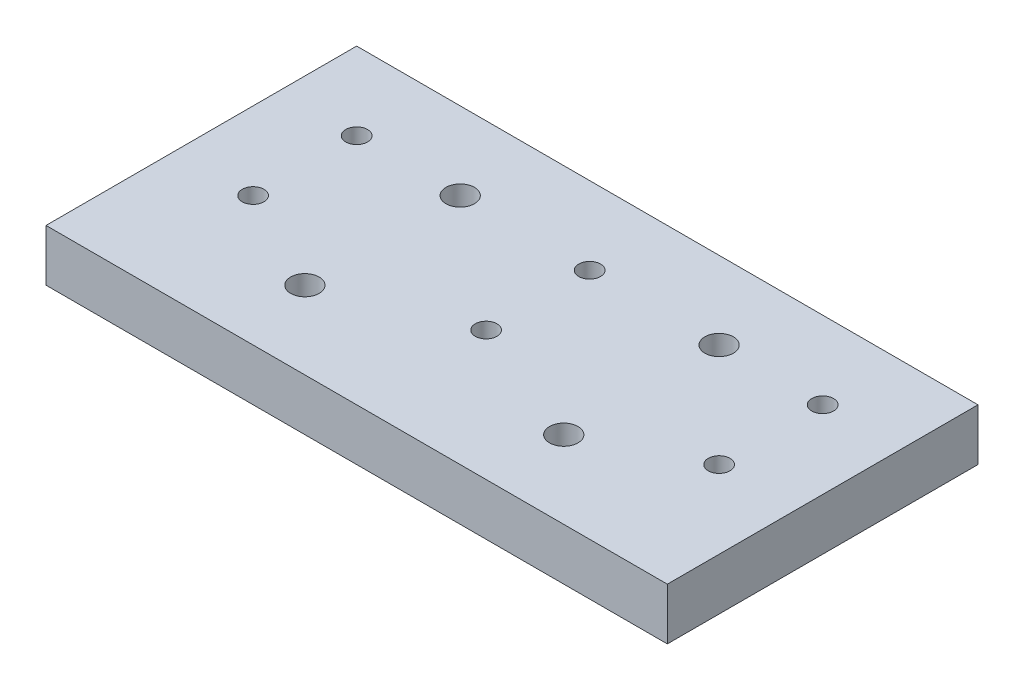
SolidWorks part; units mm, degrees
ref_plane "Front Plane" through (0, 0, 0) normal (0, 0, 1) x (1, 0, 0)
ref_plane "Top Plane" through (0, 0, 0) normal (0, 1, 0) x (1, 0, 0)
ref_plane "Right Plane" through (0, 0, 0) normal (1, 0, 0) x (0, 0, -1)
sketch "Sketch 1" plane through (0, 0, 0) normal (0, 1, 0) x (1, 0, 0)
  line L1 (-60, -30) -> (60, -30)
  line L2 (-60, -30) -> (-60, 30)
  line L3 (-60, 30) -> (60, 30)
  line L4 (60, -30) -> (60, 30)
  line L5 (-60, -30) -> (60, 30) construction
  line L6 (-60, 30) -> (60, -30) construction
  point P0 (0, 0)
  dimension "D1" = 60
  dimension "D2" = 120
extrude "Boss-Extrude 1" add sketch "Sketch 1" along normal blind 10
hole_wizard "M5 Socket Head Cap Screw Counterbore 1" positions "Sketch 3" profile "Sketch 2" counterbore size "M5" standard "JIS" end condition through all
sketch "Sketch 3" plane through (0, 0, 0) normal (0, -1, 0) x (1, 0, 0)
  point P0 (-25, 15)
  dimension "D1" = 25
  dimension "D2" = 15
sketch "Sketch 2" plane through (-25, 0, 15) normal (1, 0, 0) x (0, 0, -1)
  line L0 (0, 0) -> (0, 10)
  line L1 (0, 10) -> (2.75, 10)
  line L3 (2.75, 10) -> (2.75, 5)
  line L4 (2.75, 5) -> (5, 5)
  line L5 (5, 5) -> (5, 0)
  line L7 (5, 0) -> (0, 0)
  line L11 (0, -6.35) -> (0, 107.95) construction
  dimension "貫穿孔直徑" = 5.5
  dimension "貫穿孔深度" = 10
  dimension "柱孔直徑" = 10
  dimension "柱孔深度" = 5
pattern_linear "Linear Pattern 1" count 2 spacing 50 along (1, 0, 0) count 2 spacing 30 along (0, 0, -1) of "M5 Socket Head Cap Screw Counterbore 1"
hole_wizard "M5 Tapped Hole 1" positions "Sketch 5" profile "Sketch 4" tap size "M5" standard "GB" end condition through all
sketch "Sketch 5" plane through (0, 0, 0) normal (0, -1, 0) x (1, 0, 0)
  line L0 (-60, 30) -> (60, 30) construction
  point P0 (-45, 5)
  dimension "D1" = 45
  dimension "D2" = 25
sketch "Sketch 4" plane through (-45, 0, 5) normal (1, 0, 0) x (0, 0, -1)
  line L0 (0, 0) -> (0, 10)
  line L1 (0, 10) -> (2.1, 10)
  line L2 (2.1, 10) -> (2.1, 0)
  line L5 (2.1, 0) -> (0, 0)
  line L11 (0, -6.35) -> (0, 107.95) construction
  dimension "貫穿螺孔鑽直徑" = 4.2
  dimension "貫穿螺孔鑽深度" = 10
cosmetic thread "Cosmetic Thread 1" parameters "D2"=5
pattern_linear "Linear Pattern 2" count 2 spacing 20 along (0, 0, -1) count 3 spacing 45 along (1, 0, 0) of "M5 Tapped Hole 1"
